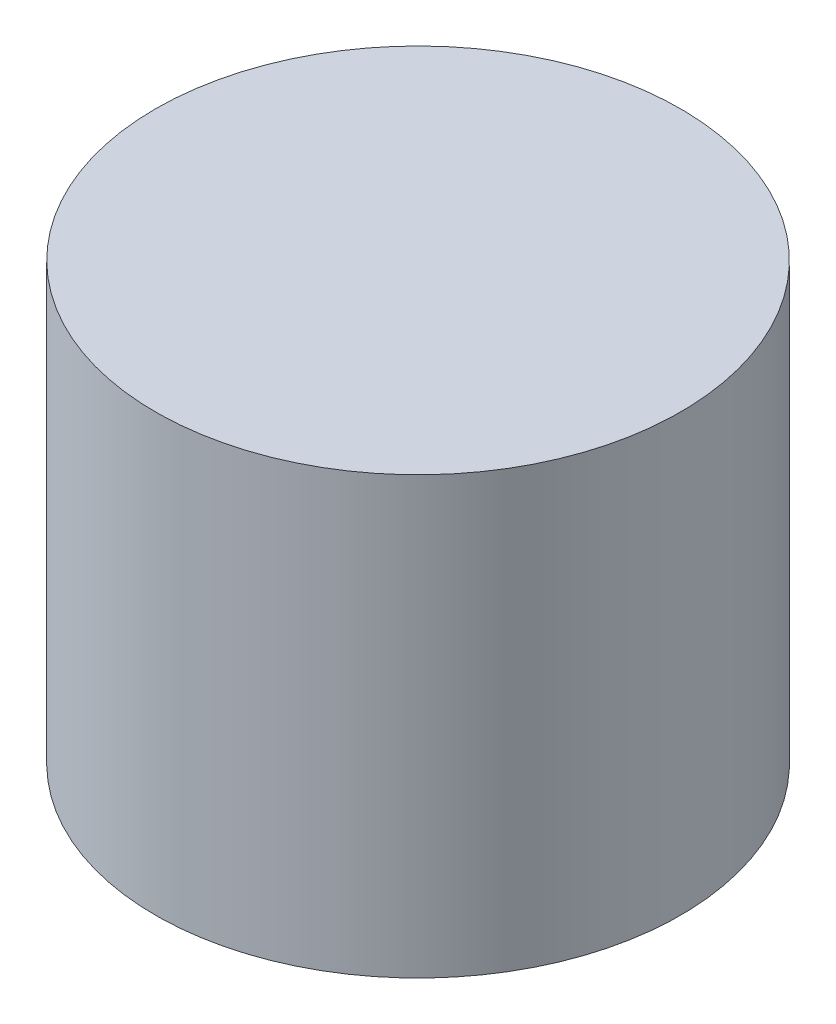
SolidWorks part; units mm, degrees
ref_plane "Front Plane" through (0, 0, 0) normal (0, 0, 1) x (1, 0, 0)
ref_plane "Top Plane" through (0, 0, 0) normal (0, 1, 0) x (1, 0, 0)
ref_plane "Right Plane" through (0, 0, 0) normal (1, 0, 0) x (0, 0, -1)
other "Configuration Table"
sketch "Sketch1" plane through (0, 0, 0) normal (0, 1, 0) x (1, 0, 0)
  circle A0 centre (0, 0) radius 8.5 construction
  circle A1 centre (0, 0) radius 8.5
sketch "Sketch2" plane through (0, 0, 0) normal (0, 0, 1) x (1, 0, 0)
  line L0 (-8.5, -0.11) -> (-8.5, 14)
  line L2 (-8.5, 14) -> (0, 14)
  line L3 (0, 14) -> (0, 0)
  line L4 (-8.5, -0.11) -> (-8, -0.11)
  line L5 (-8, -0.11) -> (-5.1016, 3.3442)
  line L6 (-5.1016, 3.3442) -> (-5.1016, 4.6658)
  line L7 (-5.1016, 4.6658) -> (-6.5, 4.6658)
  line L8 (-6.5, 4.6658) -> (-6.5, 13)
  line L9 (-6.5, 13) -> (0, 13)
  dimension "D1" = 14
  dimension "D2" = 1
  dimension "D3" = 2
  dimension "D4" = 8.5
  dimension "D5" = 0.5
  dimension "D6" = 40
  dimension "D7" = 1.3216
  dimension "D8" = 1.3984
revolve "Revolve1" add sketch "Sketch2" angle 360 about L3
